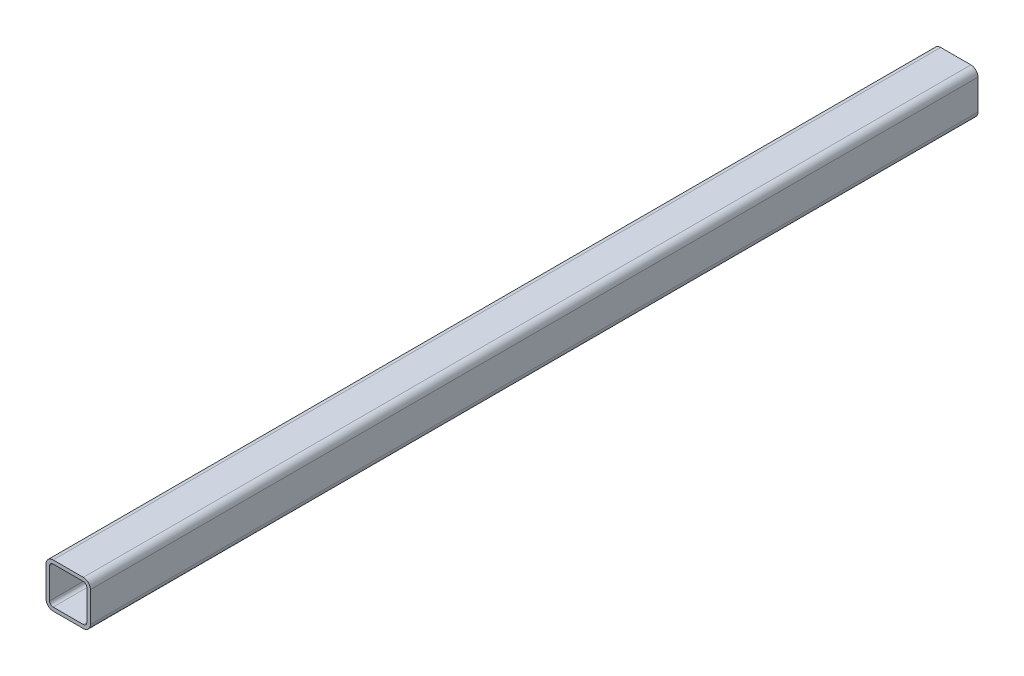
from build123d import *

# Parameters (mm, degrees)
BOSS_EXTRUDE1_DEPTH = 500


with BuildPart() as part:
    # Sketch1 → Boss-Extrude1 (new body)
    with BuildSketch(Plane.XY):
        with BuildLine():
            Line((4, 0), (21, 0))
            ThreePointArc((21, 0), (23.828427125, 1.171572875), (25, 4))
            Line((25, 4), (25, 21))
            ThreePointArc((25, 21), (23.828427125, 23.828427125), (21, 25))
            Line((21, 25), (4, 25))
            ThreePointArc((4, 25), (1.171572875, 23.828427125), (0, 21))
            Line((0, 21), (0, 4))
            ThreePointArc((0, 4), (1.171572875, 1.171572875), (4, 0))
        make_face()
        with BuildLine():
            Line((23, 4), (23, 21))
            ThreePointArc((23, 21), (22.414213562, 22.414213562), (21, 23))
            Line((21, 23), (4, 23))
            ThreePointArc((4, 23), (2.585786438, 22.414213562), (2, 21))
            Line((2, 21), (2, 4))
            ThreePointArc((2, 4), (2.585786438, 2.585786438), (4, 2))
            Line((4, 2), (21, 2))
            ThreePointArc((21, 2), (22.414213562, 2.585786438), (23, 4))
        make_face(mode=Mode.SUBTRACT)
    extrude(amount=BOSS_EXTRUDE1_DEPTH)


solid = part.part
